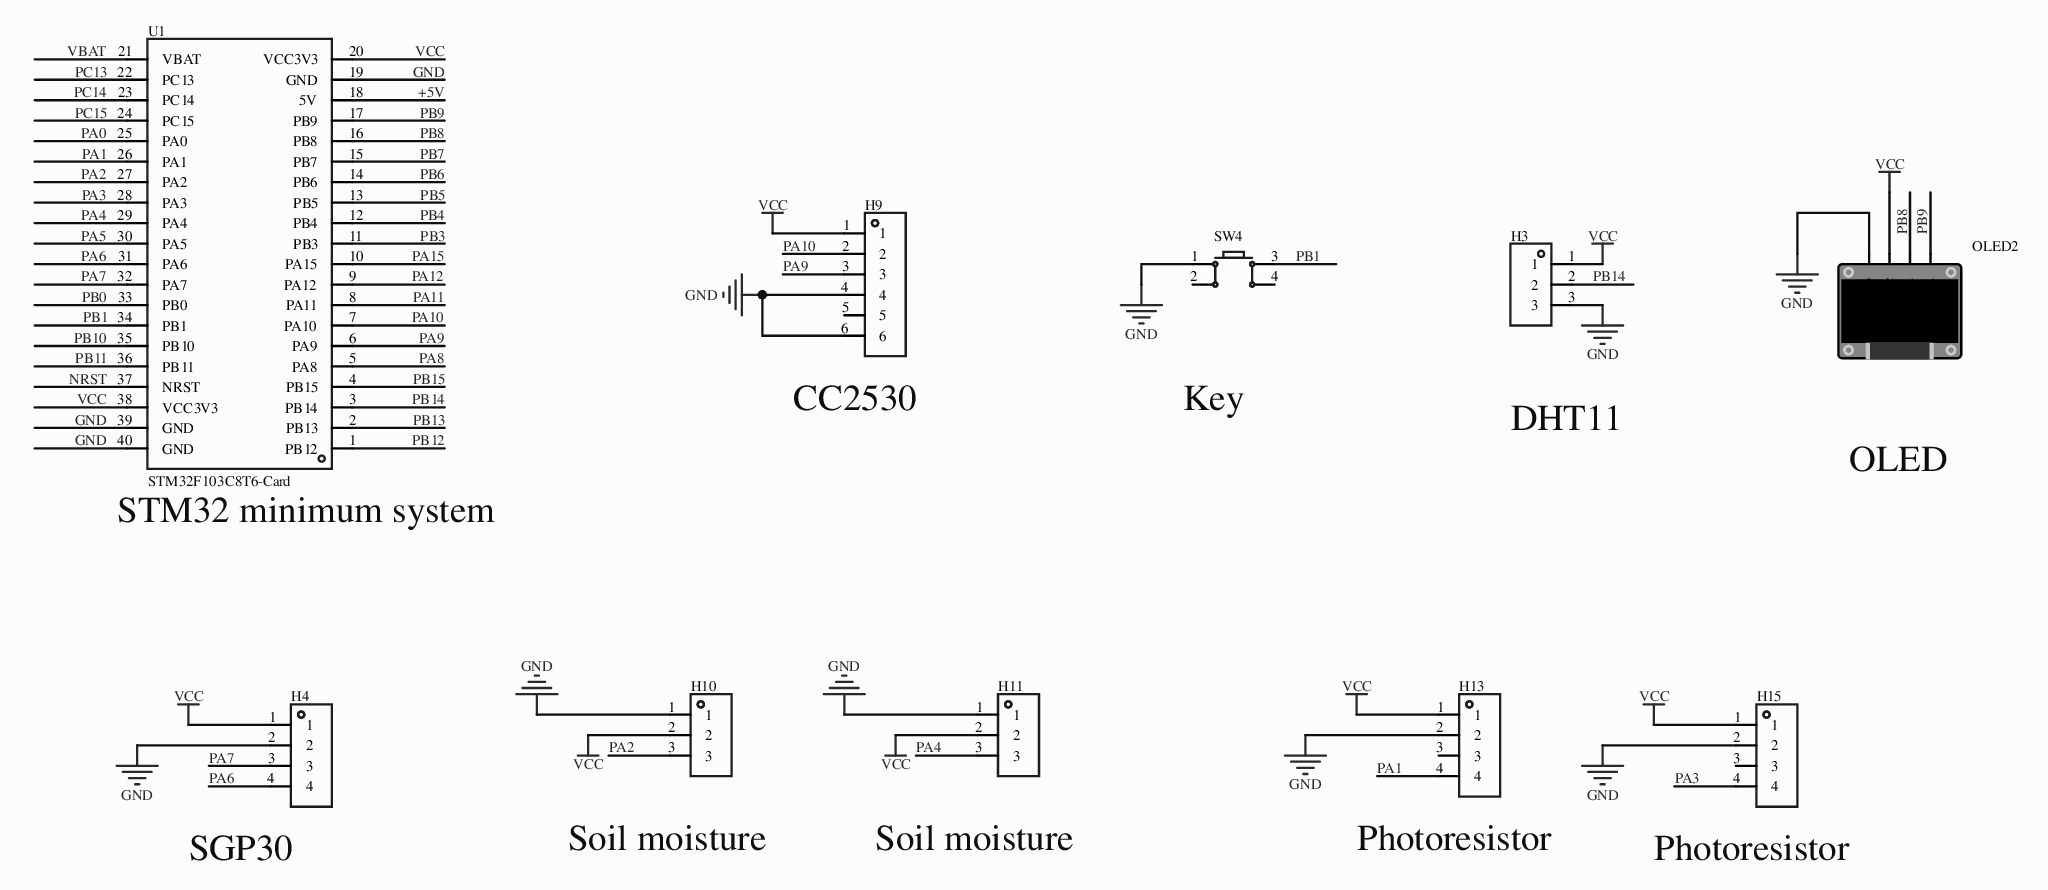
[diagram p0: MISC52023-3.schdoc]
# Altium project MISC52023-2.PrjPcb
1 sheet, 10 parts. Net scope: global (net labels, ports and power ports of the same name join across sheets).
Board file: MISC52023.pcbdoc

## Sheet MISC52023-3.schdoc
size 297 x 209 mm; Version: V1.0; @Project Name: MISC52023; @Page Count: 1; @Update Date: 2026-05-07; @Create Date: 2026-05-07; @Schematic Name: MISC52023; @Page No: 1; @Create Time: 23:22:16; @Update Time: 17:32:40; @Board Name: MISC52023

### Parts
H3  (no value)  [HDR-TH_3P-P2.54-V-F]
H4  (no value)  [HDR-TH_4P-P2.54-V-F]
H9  (no value)  [HDR-TH_6P-P2.54-V-F]
H10  (no value)  [HDR-TH_3P-P2.54-V-F]
H11  (no value)  [HDR-TH_3P-P2.54-V-F]
H13  (no value)  [HDR-TH_4P-P2.54-V-F]
H15  (no value)  [HDR-TH_4P-P2.54-V-F]
OLED2  (no value)  [0.96OLED_4P]
SW4  (no value)  [SW-TH_4P-L6.0-W6.0-P4.50-LS6.5]
U1  STM32F103C8T6-Card  [CONN-TH_L53.3-W22.9_STM32F103C8T6-CARD]

### Nets
GND: H3.3 H4.2 H9.4 H9.6 H10.1 H11.1 H13.2 H15.2 OLED2.1(GND) SW4.1 U1.19(GND) U1.39(GND) U1.40(GND)
VCC: H3.1 H4.1 H9.1 H10.2 H11.2 H13.1 H15.1 OLED2.2(VCC) U1.20(VCC3V3) U1.38(VCC3V3)
+5V: U1.18(5V)
NRST: U1.37(NRST)
PA0: U1.25(PA0)
PA1: H13.4 U1.26(PA1)
PA2: H10.3 U1.27(PA2)
PA3: H15.4 U1.28(PA3)
PA4: H11.3 U1.29(PA4)
PA5: U1.30(PA5)
PA6: H4.4 U1.31(PA6)
PA7: H4.3 U1.32(PA7)
PA8: U1.5(PA8)
PA9: H9.3 U1.6(PA9)
PA10: H9.2 U1.7(PA10)
PA11: U1.8(PA11)
PA12: U1.9(PA12)
PA15: U1.10(PA15)
PB0: U1.33(PB0)
PB1: SW4.3 U1.34(PB1)
PB3: U1.11(PB3)
PB4: U1.12(PB4)
PB5: U1.13(PB5)
PB6: U1.14(PB6)
PB7: U1.15(PB7)
PB8: OLED2.3(SCL) U1.16(PB8)
PB9: OLED2.4(SDA) U1.17(PB9)
PB10: U1.35(PB10)
PB11: U1.36(PB11)
PB12: U1.1(PB12)
PB13: U1.2(PB13)
PB14: H3.2 U1.3(PB14)
PB15: U1.4(PB15)
PC13: U1.22(PC13)
PC14: U1.23(PC14)
PC15: U1.24(PC15)
VBAT: U1.21(VBAT)

Not connected (* = marked no-connect by the designer): H9 5; H13 3; H15 3; SW4 2 4

### Notes on the sheet
- (near H9) CC2530
- Key
- (near U1) STM32 minimum system
- DHT11
- OLED
- (near H4) SGP30
- (near H10) Soil moisture
- (near H11) Soil moisture
- (near H13) Photoresistor
- (near H15) Photoresistor

### Library data of the parts
H3 = HDR-F_2.54_1x3P: Symbol: PM254V-11-03-H85; 3D Model: f3b3cc5aae9641bf9e56fc160cef875b; 3D Model Transform: 299.9994,100,0,0,0,0,0,0,-118.11; ConvertToPcb: yes; ModelName: HDR2.54-F-LI-1X3P; Device: HDR-F_2.54_1x3P; Supplier Part: C541850; Supplier Footprint: 插件; FootprintName: HDR-TH_3P-P2.54-V-F; AddInBom: yes
H4 = HDR-F_2.54_1x4P: Symbol: 2.54-1*4P female; ConvertToPcb: yes; ModelId: d187812051054f85879fcaa51a310d8e0819f05c4eef4c71ace90d822a990e87; ModelTransform: 419.6842,98.464,0,0,0,0,0,0,-118.11; Device: HDR-F_2.54_1x4P; FootprintName: HDR-TH_4P-P2.54-V-F; AddInBom: yes; SupplierPart: C2718488; Supplier Footprint: 插件; ModelName: HDR-TH_4P-P2.54-V-F
H9 = HDR-F_2.54_1x6P: Symbol: Header-Female-2.54_1x6; 3D Model: 0f5bcf94dcda47d085f24cdca1696fe9; 3D Model Transform: 619.684,94.488,0,0,0,0,0,0,-125.984; ConvertToPcb: yes; Device: HDR-F_2.54_1x6P; Supplier Part: C40877; Supplier Footprint: 插件; AddInBom: yes; FootprintName: HDR-TH_6P-P2.54-V-F; ModelName: HDR-TH_6P-P2.54-V-F
H10 H11 = HDR-F_2.54_1x3P: Symbol: PM254V-11-03-H85; ConvertToPcb: yes; ModelId: f3b3cc5aae9641bf9e56fc160cef875b; ModelName: HDR2.54-F-LI-1X3P; ModelTransform: 299.9994,100,0,0,0,0,0,0,-118.11; Device: HDR-F_2.54_1x3P; AddInBom: yes; SupplierPart: C541850; Supplier Footprint: 插件; FootprintName: HDR-TH_3P-P2.54-V-F
H13 H15 = HDR-F_2.54_1x4P: Symbol: 2.54-1*4P female; 3D Model: d187812051054f85879fcaa51a310d8e0819f05c4eef4c71ace90d822a990e87; 3D Model Transform: 419.6842,98.464,0,0,0,0,0,0,-118.11; ConvertToPcb: yes; Device: HDR-F_2.54_1x4P; Supplier Part: C2718488; Supplier Footprint: 插件; FootprintName: HDR-TH_4P-P2.54-V-F; AddInBom: yes; ModelName: HDR-TH_4P-P2.54-V-F
OLED2 = 0.96OLED模块_4P: Symbol: 0.96OLED module_4P; 3D Model: 79c000fdb68d45a296c2e9bedf4f9055; 3D Model Transform: 1393.69792,1318.895,0,0,0,0,0,-560.079,-137.795; ConvertToPcb: yes; Device: 0.96OLED module_4P; Supplier Footprint: 插件; AddInBom: yes; FootprintName: 0.96OLED_4P; ModelName: 0.96OLED_4P
SW4 = Key_TH_6x6x6: Contact current:50mA; rated voltage (DC):12V; insulation resistance:100MΩ; circuit: SPST; mounting: through-hole; button shape: round button; button/cap colour: black; actuating force:260gf@±30gf; operating temperature:-25℃~+70℃; pin style: PC pin; switch length:6mm; switch width:6mm; switch height:6mm; with bracket: no;; Symbol: Tact switch; AddInBom: yes; ModelId: 20eee248bc684ccd8cbdbb1d0d91ec6f0819f05c4eef4c71ace90d822a990e87; ModelName: SW-TH_4P-L6.0-W6.0-H5.0-LS6.5-P4.50; ModelTransform: 236.22,323.03,0,90,0,0,0,0,-137.795; Device: Key_TH_6x6x6; FootprintName: SW-TH_4P-L6.0-W6.0-P4.50-LS6.5; ConvertToPcb: yes; Supplier Footprint: 插件
U1 = STM32F103C8T6-Card: AddInBom: yes; Device: STM32F103C8T6-Card; Symbol: STM32F103C8T6-CARD; FootprintName: CONN-TH_L53.3-W22.9_STM32F103C8T6-CARD; LCSC Part Name: STM32F103C8T6-Card; SupplierPart: C9900077949; ManufacturerPart: STM32F103C8T6-Card; Supplier Footprint: 插件; Supplier: LCSC; ConvertToPcb: yes